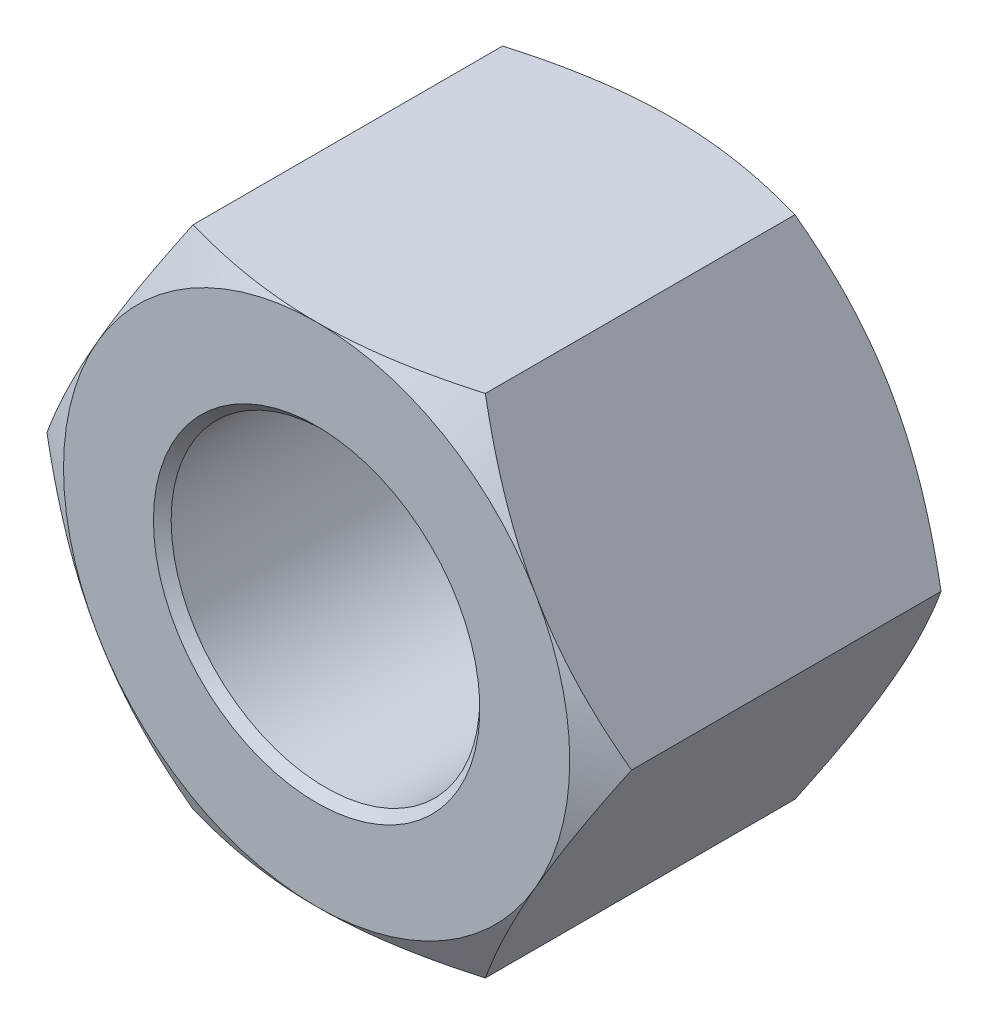
SolidWorks part; units mm, degrees
ref_plane "Plane1" through (0, 0, 0) normal (0, 0, 1) x (1, 0, 0)
ref_plane "Plane2" through (0, 0, 0) normal (0, 1, 0) x (1, 0, 0)
ref_plane "Plane3" through (0, 0, 0) normal (1, 0, 0) x (0, 0, -1)
sketch "Dimension Sketch" plane through (0, 0, 0) normal (0, 0, 1) x (1, 0, 0)
  line L0 (0, 0) -> (24, 0) construction
  point P1 (22, 0)
  point P3 (16, 0)
  point P4 (2, 0)
  point P5 (26.2, 0)
  point P6 (15.9, 0)
  point P8 (24, 0)
  dimension "D" = 16
  dimension "e(最小)" = 26.2
  dimension "m(最大)" = 15.9
  dimension "s(公称)" = 24
  dimension "dw(最小)" = 22
  dimension "P" = 2
sketch "Sketch1" plane through (0, 0, 0) normal (0, 0, 1) x (1, 0, 0)
  line L0 (-26.8088, 0) -> (37.1748, 0) construction
  line L1 (0, 25.0215) -> (0, -25.0215) construction
  line L3 (6.55, 11.3449) -> (-6.55, 11.3449)
  line L4 (-6.55, 11.3449) -> (-13.1, 0)
  line L5 (-13.1, 0) -> (-6.55, -11.3449)
  line L6 (-6.55, -11.3449) -> (6.55, -11.3449)
  line L7 (6.55, -11.3449) -> (13.1, 0)
  line L8 (13.1, 0) -> (6.55, 11.3449)
  circle A0 centre (0, 0) radius 11.3449 construction
  circle A1 centre (0, 0) radius 6.9175
  dimension "D" = 13.835
  dimension "e" = 26.2
extrude "Boss-Extrude" add sketch "Sketch1" along normal blind 15.9
cosmetic thread "Cosmetic Thread1" parameters "D2"=16
sketch "Sketch2" plane through (0, 0, 0) normal (0, 0, -1) x (-1, 0, 0)
  line L0 (-6.55, 11.3449) -> (6.55, 11.3449) construction
  circle A0 centre (0, 0) radius 11.3449
  circle A1 centre (0, 0) radius 6.9175 construction
extrude "Cut-Extrude1" cut sketch "Sketch2" against normal through all draft 60 flip side to cut
sketch "Sketch3" plane through (0, 0, 15.9) normal (0, 0, 1) x (1, 0, 0)
  line L0 (13.1, 0) -> (6.55, 11.3449) construction
  circle A0 centre (0, 0) radius 11.3449
extrude "Cut-Extrude2" cut sketch "Sketch3" against normal through all draft 60 flip side to cut
chamfer "Chamfer1" distance 0.3975 angle 45 2 edges at (6.9175, 0, 0) (6.9175, 0, 15.9)
